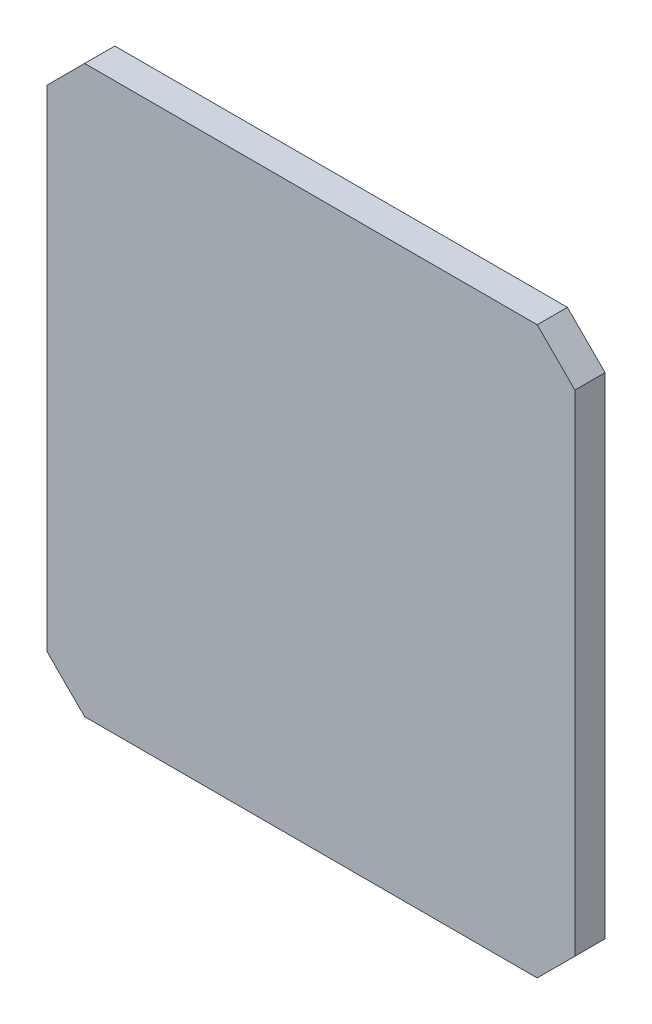
SolidWorks part; units mm, degrees
ref_plane "前视" through (0, 0, 0) normal (0, 0, 1) x (1, 0, 0)
ref_plane "上视" through (0, 0, 0) normal (0, 1, 0) x (1, 0, 0)
ref_plane "右视" through (0, 0, 0) normal (1, 0, 0) x (0, 0, -1)
sketch "草图2" plane through (0, 0, 0) normal (0, 0, 1) x (1, 0, 0)
  line L0 (0, 700) -> (50, 750)
  line L1 (50, 0) -> (650, 0)
  line L2 (0, 50) -> (0, 700)
  line L3 (50, 750) -> (650, 750)
  line L4 (700, 50) -> (700, 700)
  line L5 (650, 750) -> (700, 700)
  line L6 (50, 0) -> (0, 50)
  line L7 (650, 0) -> (700, 50)
  point P0 (0, 0)
  point P1 (700, 750)
  point P2 (0, 750)
  point P3 (700, 0)
  dimension "D1" = 700
  dimension "D2" = 750
extrude "凸台-拉伸1" add sketch "草图2" along normal blind 40
